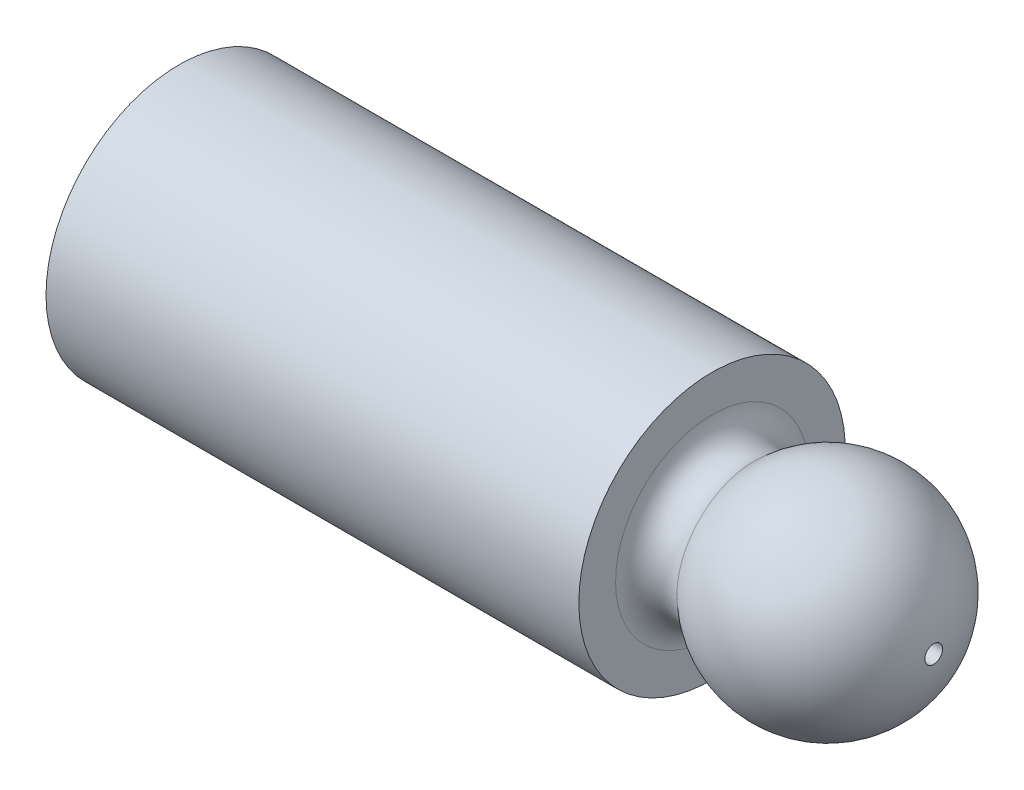
SolidWorks part; units mm, degrees
ref_plane "Front Plane" through (0, 0, 0) normal (0, 0, 1) x (1, 0, 0)
ref_plane "Top Plane" through (0, 0, 0) normal (0, 1, 0) x (1, 0, 0)
ref_plane "Right Plane" through (0, 0, 0) normal (1, 0, 0) x (0, 0, -1)
sketch "Sketch1" plane through (0, 0, 0) normal (0, 0, 1) x (1, 0, 0)
  line L0 (0, 0) -> (0, 7.5)
  line L1 (0, 7.5) -> (30, 7.5)
  line L2 (30, 7.5) -> (30, 5.4314)
  line L3 (0, 0) -> (42.5, 0) construction
  line L4 (0, 0) -> (42.5, 0)
  arc A0 (30, 5.4314) -> (32.4058, 4.386) centre (31.43, 5.4314) ccw
  arc A1 (32.4058, 4.386) -> (42.5, 0) centre (36.5, 0) cw
  dimension "D3" = 1.43
  dimension "D4" = 6
  dimension "D5" = 36.5
  dimension "D1" = 7.5
  dimension "D2" = 30
revolve "Revolve1" add sketch "Sketch1" angle 360 about L3
sketch "Sketch2" plane through (0, 0, 0) normal (0, 0, 1) x (1, 0, 0)
  line L0 (0, -16.5) -> (0, 16.5) construction
  line L1 (0, 0) -> (25, 0)
  line L2 (0, 0) -> (0, 5)
  line L3 (0, 5) -> (25, 5)
  line L4 (25, 0) -> (25, 5) construction
  line L5 (25, 0) -> (27.3094, 0)
  line L6 (25, 0) -> (25, 5) construction
  line L7 (25, 5) -> (27.3094, 1)
  line L8 (27.3094, 0) -> (27.3094, 1) construction
  line L9 (27.3094, 0) -> (37, 0)
  line L10 (27.3094, 0) -> (27.3094, 1) construction
  line L11 (27.3094, 1) -> (37, 1)
  line L12 (37, 0.5) -> (37, 1)
  line L13 (37, 0) -> (47.9541, 0)
  line L14 (37, 0) -> (37, 0.5) construction
  line L15 (37, 0.5) -> (47.9541, 0.5)
  line L16 (47.9541, 0) -> (47.9541, 0.5)
  line L17 (37, 0) -> (37, 0.5) construction
  dimension "D1" = 5
  dimension "D2" = 25
  dimension "D3" = 1
  dimension "D4" = 0.5
  dimension "D5" = 60
  dimension "D6" = 37
revolve "Cut-Revolve1" cut sketch "Sketch2" angle 360 about L1
